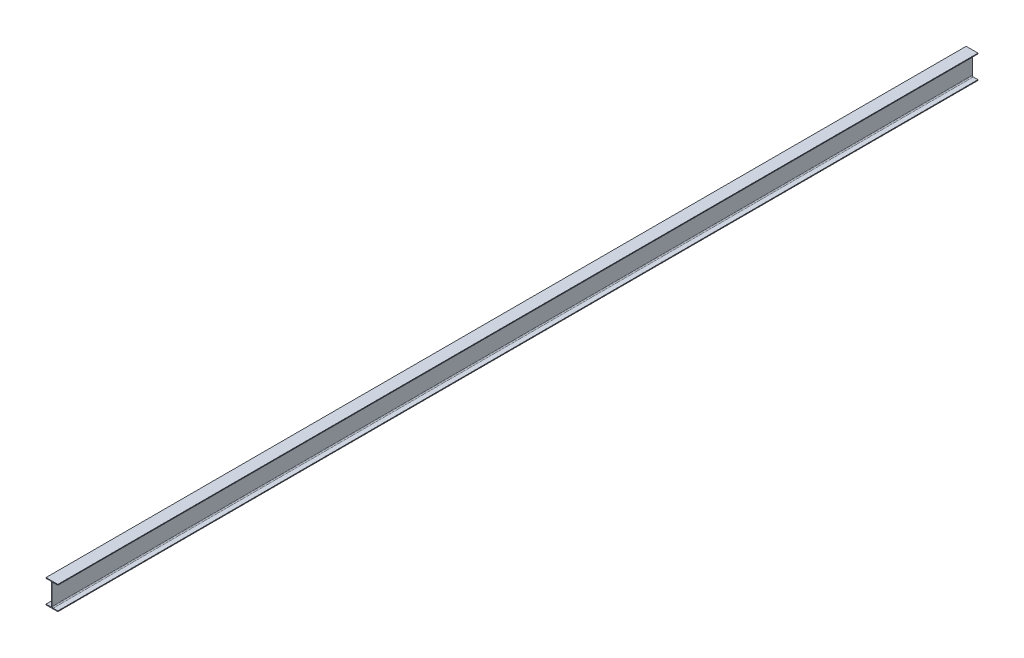
from build123d import *

# Parameters (mm, degrees)
BOSS_EXTRUDE1_DEPTH = 11647


with BuildPart() as part:
    # Sketch1 → Boss-Extrude1 (new body)
    with BuildSketch(Plane.XY):
        with BuildLine():
            Line((75, 0), (-75, 0))
            Line((-75, 0), (-75, 9))
            Line((-75, 9), (-16.25, 9))
            ThreePointArc((-16.25, 9), (-7.057611845, 12.807611845), (-3.25, 22))
            Line((-3.25, 22), (-3.25, 278))
            ThreePointArc((-3.25, 278), (-7.057611845, 287.192388155), (-16.25, 291))
            Line((-16.25, 291), (-75, 291))
            Line((-75, 291), (-75, 300))
            Line((-75, 300), (75, 300))
            Line((75, 300), (75, 291))
            Line((75, 291), (16.25, 291))
            ThreePointArc((16.25, 291), (7.057611845, 287.192388155), (3.25, 278))
            Line((3.25, 278), (3.25, 22))
            ThreePointArc((3.25, 22), (7.057611845, 12.807611845), (16.25, 9))
            Line((16.25, 9), (75, 9))
            Line((75, 9), (75, 0))
        make_face()
    extrude(amount=BOSS_EXTRUDE1_DEPTH)


solid = part.part
